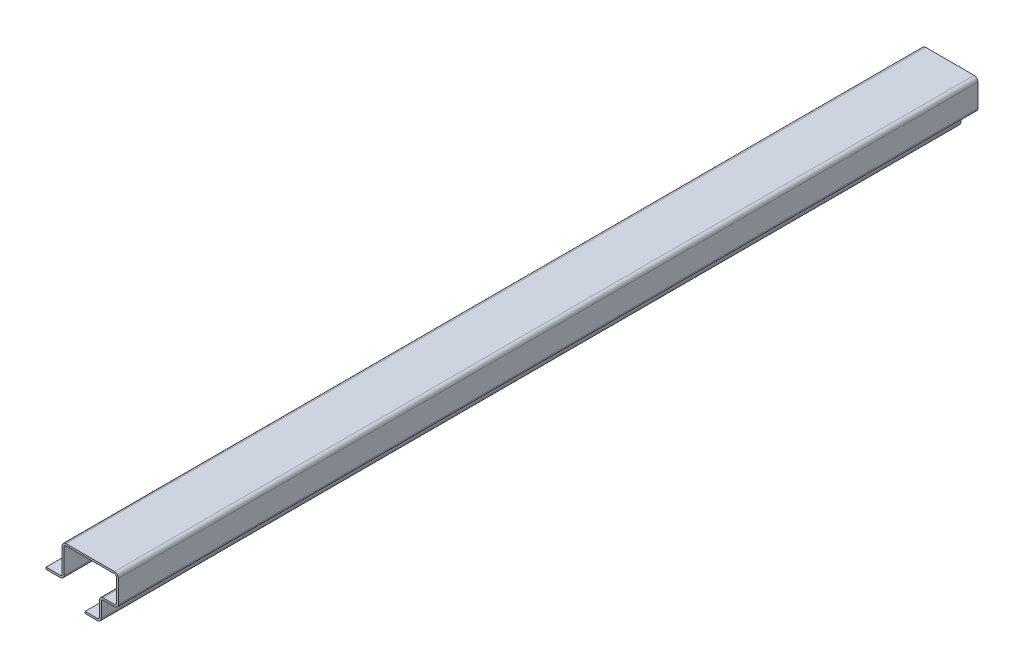
SolidWorks part; units mm, degrees
ref_plane "Front Plane" through (0, 0, 0) normal (0, 0, 1) x (1, 0, 0)
ref_plane "Top Plane" through (0, 0, 0) normal (0, 1, 0) x (1, 0, 0)
ref_plane "Right Plane" through (0, 0, 0) normal (1, 0, 0) x (0, 0, -1)
other "Configuration Table"
sketch "Sketch1" plane through (0, 0, 0) normal (0, 0, 1) x (1, 0, 0)
  line L0 (-71, 146) -> (-71, 70)
  line L1 (-77, 64) -> (-121, 64)
  line L2 (-121, 64) -> (-121, 58)
  line L3 (-121, 58) -> (-77, 58)
  line L4 (-65, 70) -> (-65, 146)
  line L5 (-59, 152) -> (91, 152)
  line L6 (97, 146) -> (97, 76)
  line L7 (91, 70) -> (56, 70)
  line L8 (44, 58) -> (44, 12)
  line L9 (38, 6) -> (0, 6)
  line L10 (0, 6) -> (0, 0)
  line L11 (0, 0) -> (38, 0)
  line L12 (50, 12) -> (50, 58)
  line L13 (56, 64) -> (91, 64)
  line L14 (103, 76) -> (103, 146)
  line L15 (91, 158) -> (-59, 158)
  arc A0 (-59, 158) -> (-71, 146) centre (-59, 146) ccw
  arc A1 (-77, 64) -> (-71, 70) centre (-77, 70) ccw
  arc A2 (-77, 58) -> (-65, 70) centre (-77, 70) ccw
  arc A3 (-59, 152) -> (-65, 146) centre (-59, 146) ccw
  arc A4 (97, 146) -> (91, 152) centre (91, 146) ccw
  arc A5 (91, 70) -> (97, 76) centre (91, 76) ccw
  arc A6 (56, 70) -> (44, 58) centre (56, 58) ccw
  arc A7 (38, 6) -> (44, 12) centre (38, 12) ccw
  arc A8 (38, 0) -> (50, 12) centre (38, 12) ccw
  arc A9 (56, 64) -> (50, 58) centre (56, 58) ccw
  arc A10 (91, 64) -> (103, 76) centre (91, 76) ccw
  arc A11 (103, 146) -> (91, 158) centre (91, 146) ccw
  dimension "D1" = 12
  dimension "D2" = 44
  dimension "D3" = 97
  dimension "D4" = 65
  dimension "D5" = 121
  dimension "D6" = 58
  dimension "D7" = 152
extrude "Boss-Extrude1" add sketch "Sketch1" along normal blind 2660
